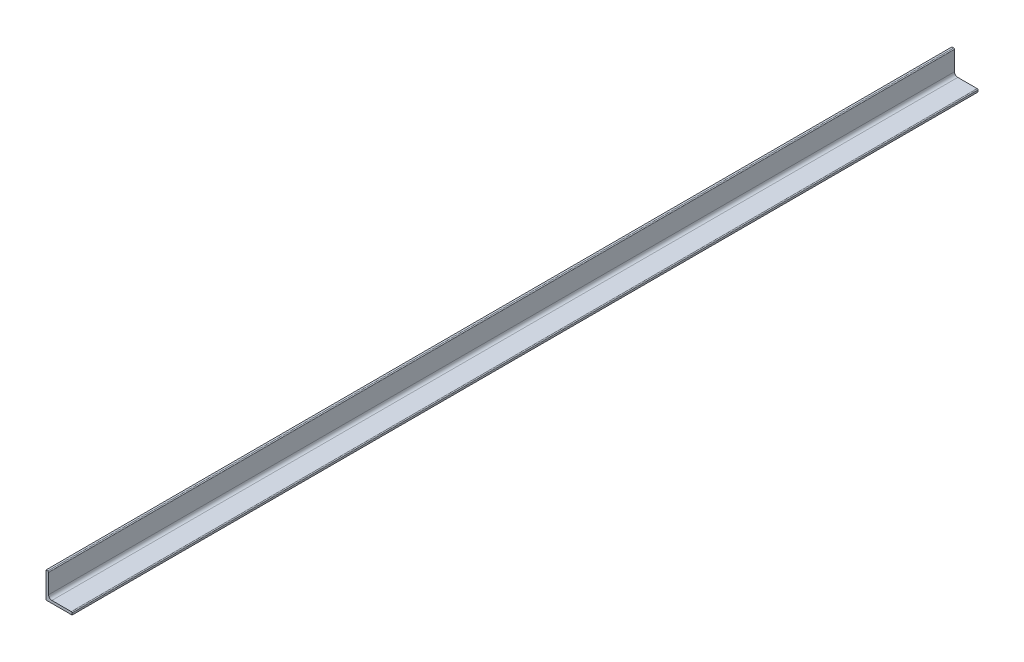
SolidWorks part; units mm, degrees
material "Q235B"
ref_plane "Plane1" through (0, 0, 0) normal (0, 0, 1) x (1, 0, 0)
ref_plane "Plane2" through (0, 0, 0) normal (0, 1, 0) x (1, 0, 0)
ref_plane "Plane3" through (0, 0, 0) normal (1, 0, 0) x (0, 0, -1)
sketch "Sketch1" plane through (0, 0, 0) normal (0, 0, 1) x (1, 0, 0)
  line L0 (0, 0) -> (0, 40)
  line L1 (0, 20) -> (4, 20) construction
  line L2 (4, 38.6667) -> (4, 9)
  line L3 (9, 4) -> (38.6667, 4)
  line L4 (20, 4) -> (20, 0) construction
  line L5 (40, 0) -> (0, 0)
  line L6 (0, 40) -> (2.6667, 40)
  line L7 (40, 0) -> (40, 2.6667)
  arc A0 (40, 2.6667) -> (38.6667, 4) centre (38.6667, 2.6667) ccw
  arc A1 (2.6667, 40) -> (4, 38.6667) centre (2.6667, 38.6667) cw
  arc A2 (9, 4) -> (4, 9) centre (9, 9) cw
  point P10 (20, 0)
  point P14 (0, 20)
  point P15 (4, 20)
  point P16 (20, 4)
  point P17 (4, 40)
  point P18 (40, 4)
  point P21 (40, 4)
  point P24 (4, 40)
extrude "Boss-Extrude1" add sketch "Sketch1" along normal blind 1389 contours L3 A0 L7 L5 L0 L6 A1 L2 A2
equation "\"D2@Sketch1\" = \"D1@Sketch1\" / 3"
